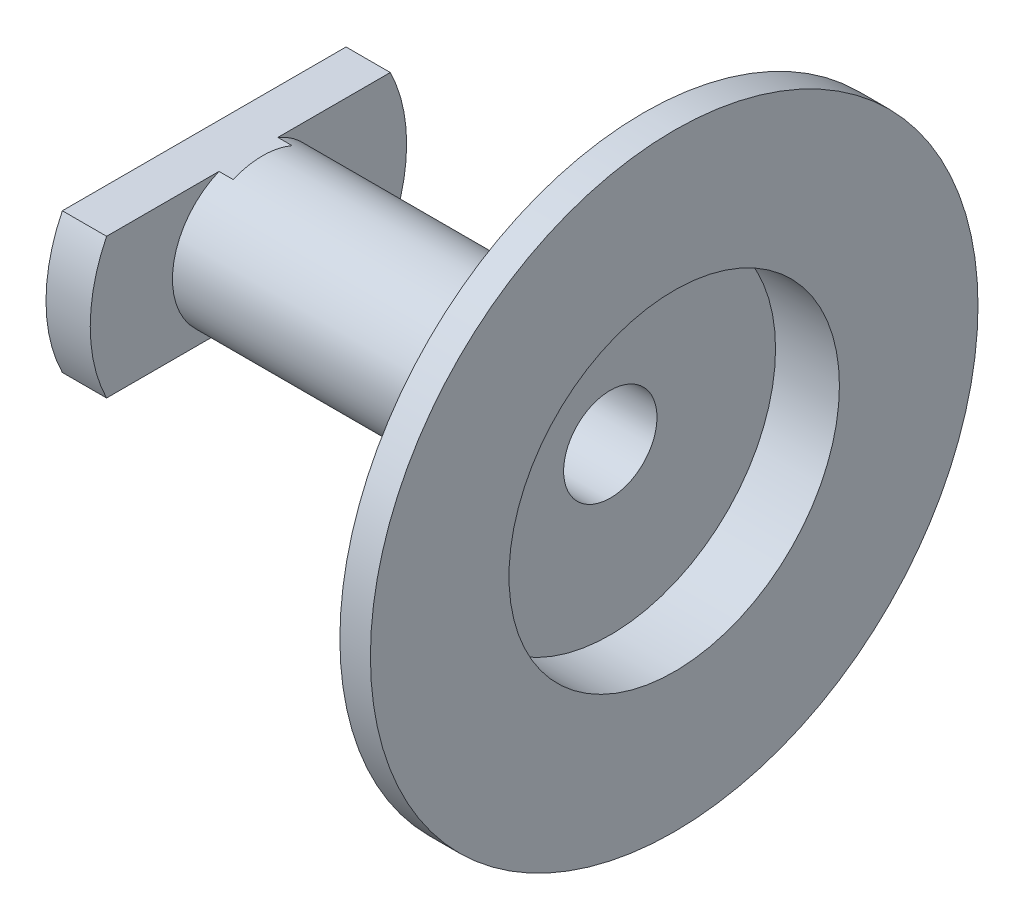
from build123d import *

# Parameters (mm, degrees)
SKETCH2_W          = 82.566044685
SKETCH2_H          = 15.592809798
SKETCH2_W_2        = 148.96712198
SKETCH2_H_2        = 11.958140401
CUT_EXTRUDE1_DEPTH = 5


with BuildPart() as part:
    # Sketch1 → Revolve1 (revolve)
    with BuildSketch(Plane.XY, mode=Mode.PRIVATE) as revolve1_sk:
        Polygon((-74.14259961, 26.024332396), (-74.14259961, 17.45458405), (-79.306985444, 17.45458405), (-79.306985444, 6.508165042), (-108, 6.508165042), (-108, 13.551665989), (-109.954236571, 13.551665989), (-111.789002112, 13.551665989), (-111.789002112, 4), (-106.267464057, 4), (-77, 4), (-77, 14.153673902), (-71.527344849, 14.153673902), (-71.527344849, 26.024332396), align=None)
    revolve(revolve1_sk.sketch.rotate(Axis((0, 0, 0), (-1, 0, 0)), 90), axis=Axis((0, 0, 0), (-1, 0, 0)))

    # Sketch2 → Cut-Extrude1 (cut)
    with BuildSketch(Plane.ZY.offset(111.789002112)):
        with Locations((-3.321091868, 13.796404899)):
            Rectangle(SKETCH2_W, SKETCH2_H)
        with Locations((5.512682346, -11.979070201)):
            Rectangle(SKETCH2_W_2, SKETCH2_H_2)
    extrude(amount=-CUT_EXTRUDE1_DEPTH, mode=Mode.SUBTRACT)


solid = part.part
